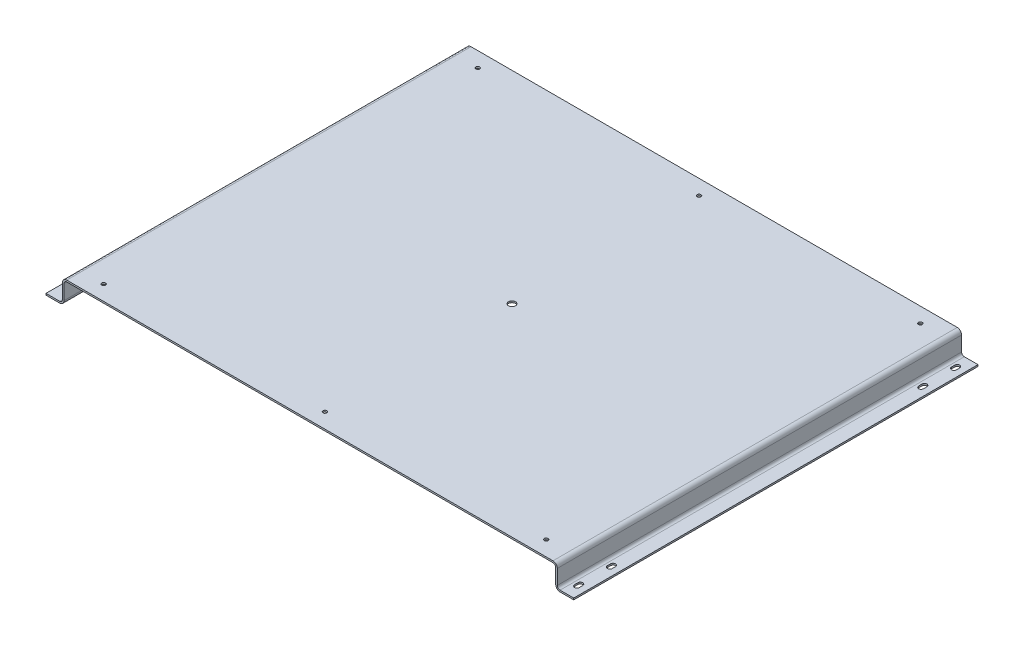
from build123d import *

# Parameters (mm, degrees)
EXTRUDE_1_DEPTH     = 740
SKETCH_2_R          = 3.5
CUT_EXTRUDE_1_DEPTH = 740
CUT_EXTRUDE_2_DEPTH = 740
SKETCH_4_R          = 6.5
CUT_EXTRUDE_3_DEPTH = 10


with BuildPart() as part:
    # 草图1 → 凸台-拉伸1 (new body)
    with BuildSketch(Plane.XY):
        with BuildLine():
            Line((0, 0), (25, 0))
            ThreePointArc((25, 0), (30.656854249, 2.343145751), (33, 8))
            Line((33, 8), (33, 35))
            ThreePointArc((33, 35), (34.464466094, 38.535533906), (38, 40))
            Line((38, 40), (928, 40))
            ThreePointArc((928, 40), (931.535533906, 38.535533906), (933, 35))
            Line((933, 35), (933, 8))
            ThreePointArc((933, 8), (935.343145751, 2.343145751), (941, 0))
            Line((941, 0), (966, 0))
            Line((966, 0), (966, 3))
            Line((966, 3), (941, 3))
            ThreePointArc((941, 3), (937.464466094, 4.464466094), (936, 8))
            Line((936, 8), (936, 35))
            ThreePointArc((936, 35), (933.656854249, 40.656854249), (928, 43))
            Line((928, 43), (38, 43))
            ThreePointArc((38, 43), (32.343145751, 40.656854249), (30, 35))
            Line((30, 35), (30, 8))
            ThreePointArc((30, 8), (28.535533906, 4.464466094), (25, 3))
            Line((25, 3), (0, 3))
            Line((0, 3), (0, 0))
        make_face()
    extrude(amount=EXTRUDE_1_DEPTH)

    # 草图2 → 切除-拉伸1 (cut)
    with BuildSketch(Plane(origin=(0, 43, 0), x_dir=(1, 0, 0), z_dir=(0, 1, 0))):
        with Locations(Location((78, -27.5, 0), (0, 0, 180))):
            Circle(SKETCH_2_R)
        with Locations(Location((483, -27.5, 0), (0, 0, 180))):
            Circle(SKETCH_2_R)
        with Locations(Location((888, -27.5, 0), (0, 0, 180))):
            Circle(SKETCH_2_R)
        with Locations(Location((78, -712.5, 0), (0, 0, 180))):
            Circle(SKETCH_2_R)
        with Locations(Location((888, -712.5, 0), (0, 0, 180))):
            Circle(SKETCH_2_R)
        with Locations(Location((483, -712.5, 0), (0, 0, 180))):
            Circle(SKETCH_2_R)
    extrude(amount=-CUT_EXTRUDE_1_DEPTH, mode=Mode.SUBTRACT)

    # 草图3 → 切除-拉伸2 (cut)
    with BuildSketch(Plane(origin=(0, 3, 0), x_dir=(1, 0, 0), z_dir=(0, 1, 0))):
        with BuildLine():
            Line((20.5, -22), (20.5, -28))
            ThreePointArc((20.5, -28), (16, -32.5), (11.5, -28))
            Line((11.5, -28), (11.5, -22))
            ThreePointArc((11.5, -22), (16, -17.5), (20.5, -22))
        make_face()
        with BuildLine():
            Line((20.5, -82), (20.5, -88))
            ThreePointArc((20.5, -88), (16, -92.5), (11.5, -88))
            Line((11.5, -88), (11.5, -82))
            ThreePointArc((11.5, -82), (16, -77.5), (20.5, -82))
        make_face()
        with BuildLine():
            Line((945.5, -82), (945.5, -88))
            ThreePointArc((945.5, -88), (950, -92.5), (954.5, -88))
            Line((954.5, -88), (954.5, -82))
            ThreePointArc((954.5, -82), (950, -77.5), (945.5, -82))
        make_face()
        with BuildLine():
            Line((945.5, -22), (945.5, -28))
            ThreePointArc((945.5, -28), (950, -32.5), (954.5, -28))
            Line((954.5, -28), (954.5, -22))
            ThreePointArc((954.5, -22), (950, -17.5), (945.5, -22))
        make_face()
        with BuildLine():
            Line((945.5, -658), (945.5, -652))
            ThreePointArc((945.5, -652), (950, -647.5), (954.5, -652))
            Line((954.5, -652), (954.5, -658))
            ThreePointArc((954.5, -658), (950, -662.5), (945.5, -658))
        make_face()
        with BuildLine():
            Line((945.5, -718), (945.5, -712))
            ThreePointArc((945.5, -712), (950, -707.5), (954.5, -712))
            Line((954.5, -712), (954.5, -718))
            ThreePointArc((954.5, -718), (950, -722.5), (945.5, -718))
        make_face()
        with BuildLine():
            Line((20.5, -658), (20.5, -652))
            ThreePointArc((20.5, -652), (16, -647.5), (11.5, -652))
            Line((11.5, -652), (11.5, -658))
            ThreePointArc((11.5, -658), (16, -662.5), (20.5, -658))
        make_face()
        with BuildLine():
            Line((20.5, -718), (20.5, -712))
            ThreePointArc((20.5, -712), (16, -707.5), (11.5, -712))
            Line((11.5, -712), (11.5, -718))
            ThreePointArc((11.5, -718), (16, -722.5), (20.5, -718))
        make_face()
    extrude(amount=-CUT_EXTRUDE_2_DEPTH, mode=Mode.SUBTRACT)

    # 草图4 → 切除-拉伸3 (cut)
    with BuildSketch(Plane(origin=(0, 43, 0), x_dir=(1, 0, 0), z_dir=(0, 1, 0))):
        with Locations(Location((483, -370, 0), (0, 0, 180))):
            Circle(SKETCH_4_R)
    extrude(amount=-CUT_EXTRUDE_3_DEPTH, mode=Mode.SUBTRACT)


solid = part.part
